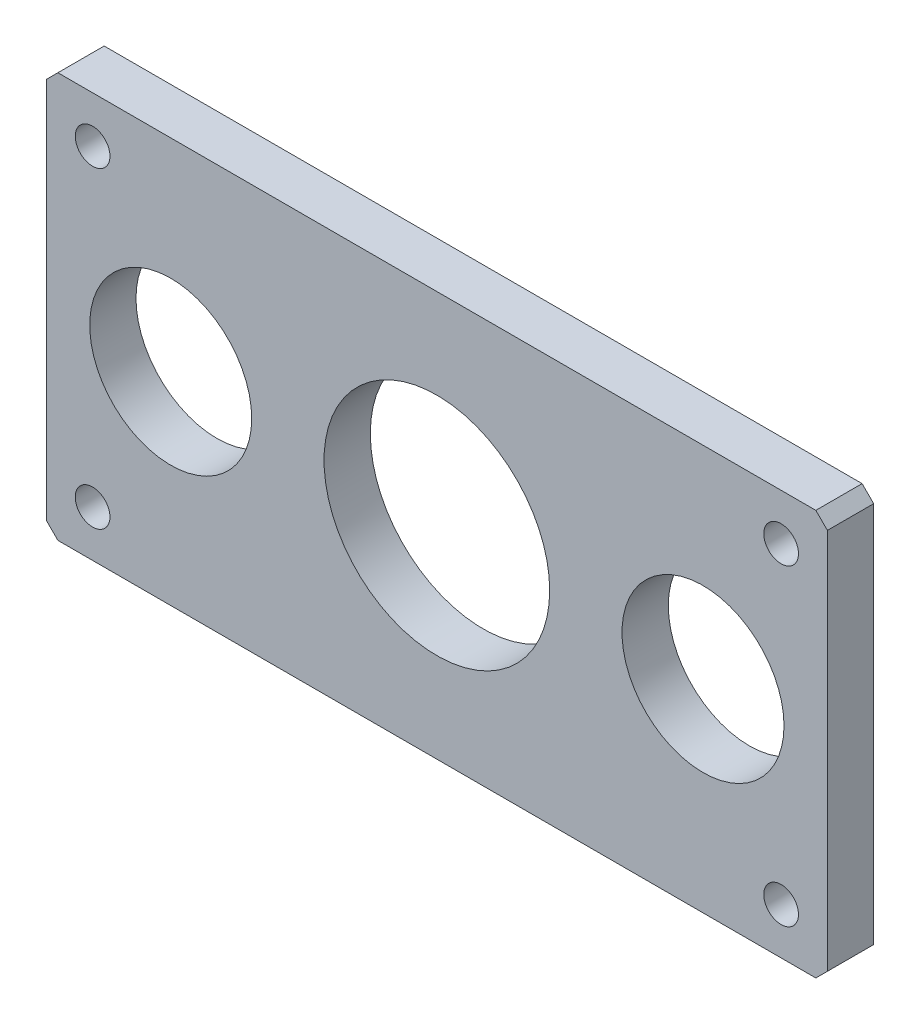
from build123d import *

# Parameters (mm, degrees)
SKETCH_1_W          = 135
SKETCH_1_H          = 70
EXTRUDE_1_DEPTH     = 8
CUT_EXTRUDE_1_REACH = 78.454
SKETCH_2_R          = 19.5
CUT_EXTRUDE_2_REACH = 78.454
SKETCH_3_R          = 14
CUT_EXTRUDE_3_REACH = 78.454
SKETCH_4_R          = 3
CHAMFER_1_SIZE      = 2


with BuildPart() as part:
    # 草图1 → 凸台-拉伸1 (new body)
    with BuildSketch(Plane.XY):
        Rectangle(SKETCH_1_W, SKETCH_1_H)
    extrude(amount=EXTRUDE_1_DEPTH)

    # 草图2 → 切除-拉伸1 (cut, up to next)
    with BuildSketch(Plane.XY.offset(8), mode=Mode.PRIVATE) as cut_extrude_1_sk1:
        Circle(SKETCH_2_R)
    cut_extrude_1_tool1 = extrude(cut_extrude_1_sk1.sketch, amount=-CUT_EXTRUDE_1_REACH, mode=Mode.PRIVATE) & part.part
    add(cut_extrude_1_tool1.solids().sort_by_distance((0, 0, 8))[0], mode=Mode.SUBTRACT)

    # 草图3 → 切除-拉伸2 (cut, up to next)
    with BuildSketch(Plane.XY.offset(8), mode=Mode.PRIVATE) as cut_extrude_2_sk1:
        with Locations((46, 0)):
            Circle(SKETCH_3_R)
    cut_extrude_2_tool1 = extrude(cut_extrude_2_sk1.sketch, amount=-CUT_EXTRUDE_2_REACH, mode=Mode.PRIVATE) & part.part
    # 草图3 → 切除-拉伸2 (cut, up to next)
    with BuildSketch(Plane.XY.offset(8), mode=Mode.PRIVATE) as cut_extrude_2_sk2:
        with Locations((-46, 0)):
            Circle(SKETCH_3_R)
    cut_extrude_2_tool2 = extrude(cut_extrude_2_sk2.sketch, amount=-CUT_EXTRUDE_2_REACH, mode=Mode.PRIVATE) & part.part
    add(cut_extrude_2_tool1.solids().sort_by_distance((46, 0, 8))[0], mode=Mode.SUBTRACT)
    add(cut_extrude_2_tool2.solids().sort_by_distance((-46, 0, 8))[0], mode=Mode.SUBTRACT)

    # 草图4 → 切除-拉伸3 (cut, up to next)
    with BuildSketch(Plane.XY.offset(8), mode=Mode.PRIVATE) as cut_extrude_3_sk1:
        with Locations((-59.5, 27)):
            Circle(SKETCH_4_R)
    cut_extrude_3_tool1 = extrude(cut_extrude_3_sk1.sketch, amount=-CUT_EXTRUDE_3_REACH, mode=Mode.PRIVATE) & part.part
    # 草图4 → 切除-拉伸3 (cut, up to next)
    with BuildSketch(Plane.XY.offset(8), mode=Mode.PRIVATE) as cut_extrude_3_sk2:
        with Locations((-59.5, -27)):
            Circle(SKETCH_4_R)
    cut_extrude_3_tool2 = extrude(cut_extrude_3_sk2.sketch, amount=-CUT_EXTRUDE_3_REACH, mode=Mode.PRIVATE) & part.part
    # 草图4 → 切除-拉伸3 (cut, up to next)
    with BuildSketch(Plane.XY.offset(8), mode=Mode.PRIVATE) as cut_extrude_3_sk3:
        with Locations(Location((59.5, -27, 0), (0, 0, 180))):
            Circle(SKETCH_4_R)
    cut_extrude_3_tool3 = extrude(cut_extrude_3_sk3.sketch, amount=-CUT_EXTRUDE_3_REACH, mode=Mode.PRIVATE) & part.part
    # 草图4 → 切除-拉伸3 (cut, up to next)
    with BuildSketch(Plane.XY.offset(8), mode=Mode.PRIVATE) as cut_extrude_3_sk4:
        with Locations(Location((59.5, 27, 0), (0, 0, 180))):
            Circle(SKETCH_4_R)
    cut_extrude_3_tool4 = extrude(cut_extrude_3_sk4.sketch, amount=-CUT_EXTRUDE_3_REACH, mode=Mode.PRIVATE) & part.part
    add(cut_extrude_3_tool1.solids().sort_by_distance((-59.5, 27, 8))[0], mode=Mode.SUBTRACT)
    add(cut_extrude_3_tool2.solids().sort_by_distance((-59.5, -27, 8))[0], mode=Mode.SUBTRACT)
    add(cut_extrude_3_tool3.solids().sort_by_distance((59.5, -27, 8))[0], mode=Mode.SUBTRACT)
    add(cut_extrude_3_tool4.solids().sort_by_distance((59.5, 27, 8))[0], mode=Mode.SUBTRACT)

    # 倒角1
    chamfer_1_edges = [part.edges().sort_by_distance(p)[0] for p in [
        (67.5, -35, 4),
        (-67.5, -35, 4),
        (-67.5, 35, 4),
        (67.5, 35, 4),
    ]]
    chamfer(chamfer_1_edges, length=CHAMFER_1_SIZE)


solid = part.part
